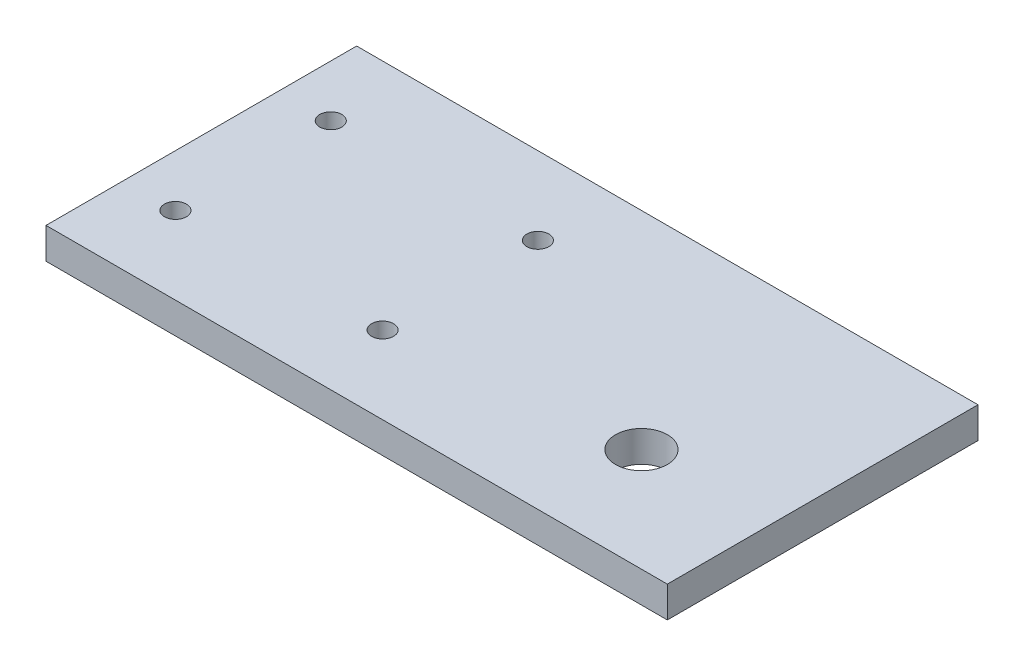
from build123d import *

# Parameters (mm, degrees)
SKETCH_1_W      = 240
SKETCH_1_H      = 120
SKETCH_1_R      = 4.25
SKETCH_1_R_2    = 10
EXTRUDE_1_DEPTH = 12


with BuildPart() as part:
    # 草图1 → 凸台-拉伸1 (new body)
    with BuildSketch(Plane(origin=(0, 0, 0), x_dir=(1, 0, 0), z_dir=(0, 1, 0))):
        with Locations((120, 60)):
            Rectangle(SKETCH_1_W, SKETCH_1_H)
        with Locations(Location((20, 30, 0), (0, 0, 270))):
            Circle(SKETCH_1_R, mode=Mode.SUBTRACT)
        with Locations(Location((20, 90, 0), (0, 0, 270))):
            Circle(SKETCH_1_R, mode=Mode.SUBTRACT)
        with Locations(Location((100, 90, 0), (0, 0, 270))):
            Circle(SKETCH_1_R, mode=Mode.SUBTRACT)
        with Locations(Location((100, 30, 0), (0, 0, 270))):
            Circle(SKETCH_1_R, mode=Mode.SUBTRACT)
        with Locations(Location((190, 40, 0), (0, 0, 270))):
            Circle(SKETCH_1_R_2, mode=Mode.SUBTRACT)
    extrude(amount=EXTRUDE_1_DEPTH)


solid = part.part
